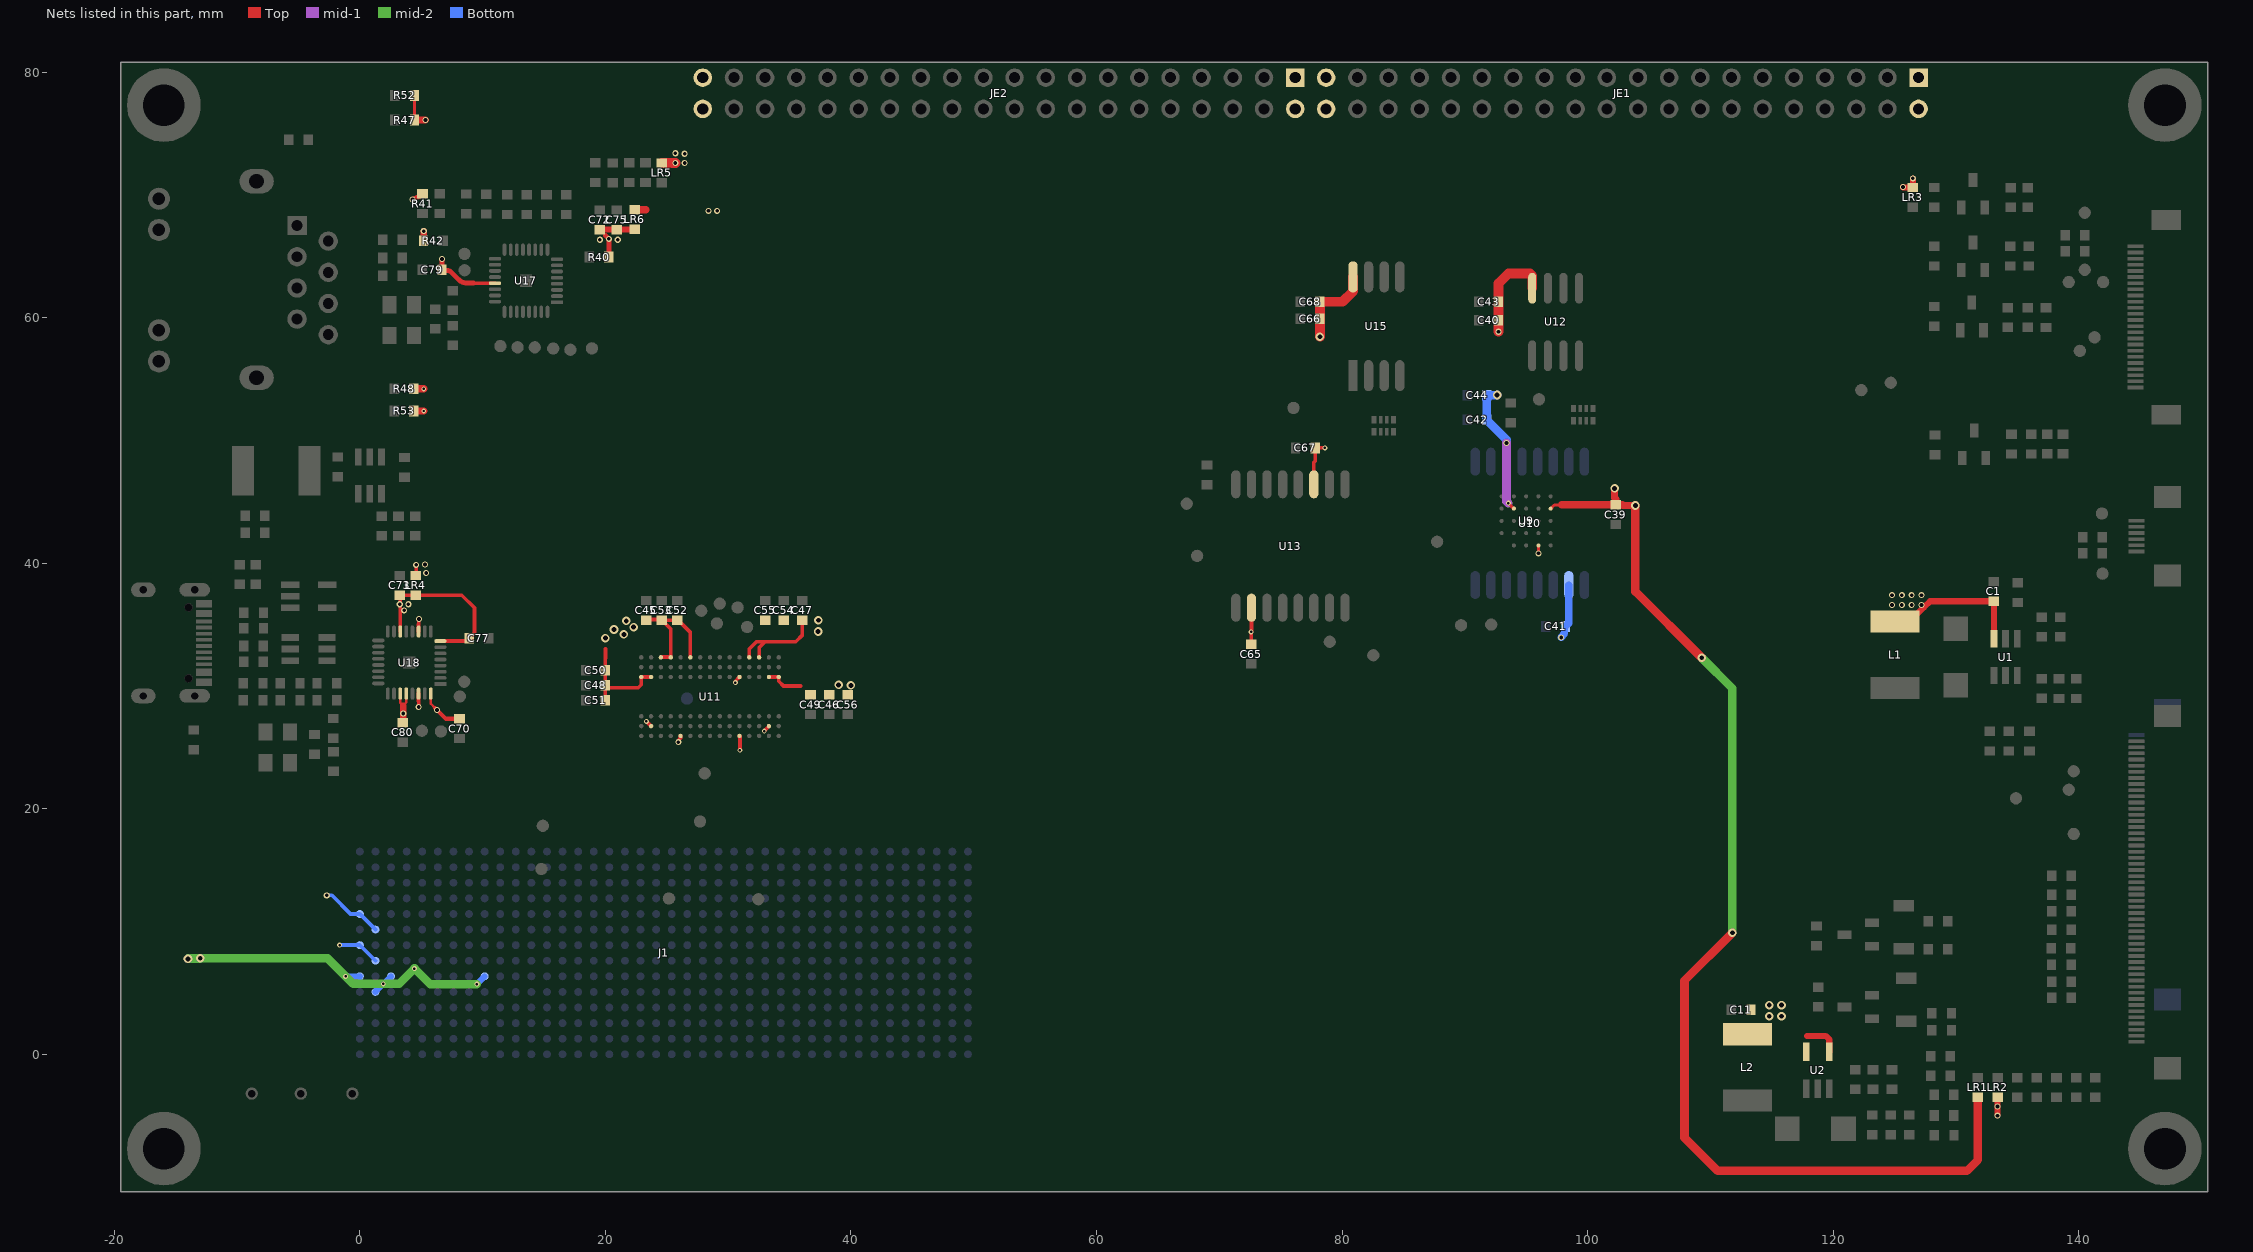
[diagram p0: the nets of this part, all layers, seen from the top]
# Altium PCB MISC105414.PcbDoc (part 3 of 11)
Units mm, origin at the board's own origin, x right, y up, seen from the top; angles counter-clockwise.
Board outline 170 x 92 mm, 6 copper layers (Top, GND, mid-1, mid-2, mid-3, Bottom), stack 1.231 mm thick; 238 components, 304 nets, 1456 pads, 1258 vias.
Unrouted connection lines stored in the file: 57.

## Footprints (in the part's own frame and the unit in brackets; to place one, negate y for a bottom-side part, rotate by r counter-clockwise, add the part's x,y. Pads: shape width x height; smd on the part's side, far side on the other; paste and mask are expansions set on the pad) (continued)
ASP-184330-01_BOTTOM [mm]
  round 0.64 smd far side: A1(0,-2.54) A2(1.27,-2.54) A3(2.54,-2.54) A4(3.81,-2.54) A5(5.08,-2.54) A6(6.35,-2.54) A7(7.62,-2.54) A8(8.89,-2.54) A9(10.16,-2.54) A10(11.43,-2.54) A11(12.7,-2.54) A12(13.97,-2.54) A13(15.24,-2.54) A14(16.51,-2.54) A15(17.78,-2.54) A16(19.05,-2.54) A17(20.32,-2.54) A18(21.59,-2.54) A19(22.86,-2.54) A20(24.13,-2.54) A21(25.4,-2.54) A22(26.67,-2.54) A23(27.94,-2.54) A24(29.21,-2.54) A25(30.48,-2.54) A26(31.75,-2.54) A27(33.02,-2.54) A28(34.29,-2.54) A29(35.56,-2.54) A30(36.83,-2.54) A31(38.1,-2.54) A32(39.37,-2.54) A33(40.64,-2.54) A34(41.91,-2.54) A35(43.18,-2.54) A36(44.45,-2.54) A37(45.72,-2.54) A38(46.99,-2.54) A39(48.26,-2.54) A40(49.53,-2.54) B1(0,-3.81) B2(1.27,-3.81) B3(2.54,-3.81) B4(3.81,-3.81) B5(5.08,-3.81) B6(6.35,-3.81) B7(7.62,-3.81) B8(8.89,-3.81) B9(10.16,-3.81) B10(11.43,-3.81) B11(12.7,-3.81) B12(13.97,-3.81) B13(15.24,-3.81) B14(16.51,-3.81) B15(17.78,-3.81) B16(19.05,-3.81) B17(20.32,-3.81) B18(21.59,-3.81) B19(22.86,-3.81) B20(24.13,-3.81) B21(25.4,-3.81) B22(26.67,-3.81) B23(27.94,-3.81) B24(29.21,-3.81) B25(30.48,-3.81) B26(31.75,-3.81) B27(33.02,-3.81) B28(34.29,-3.81) B29(35.56,-3.81) B30(36.83,-3.81) B31(38.1,-3.81) B32(39.37,-3.81) B33(40.64,-3.81) B34(41.91,-3.81) B35(43.18,-3.81) B36(44.45,-3.81) B37(45.72,-3.81) B38(46.99,-3.81) B39(48.26,-3.81) B40(49.53,-3.81) C1(0,-5.08) C2(1.27,-5.08) C3(2.54,-5.08) C4(3.81,-5.08) C5(5.08,-5.08) C6(6.35,-5.08) C7(7.62,-5.08) C8(8.89,-5.08) C9(10.16,-5.08) C10(11.43,-5.08) C11(12.7,-5.08) C12(13.97,-5.08) C13(15.24,-5.08) C14(16.51,-5.08) C15(17.78,-5.08) C16(19.05,-5.08) C17(20.32,-5.08) C18(21.59,-5.08) C19(22.86,-5.08) C20(24.13,-5.08) C21(25.4,-5.08) C22(26.67,-5.08) C23(27.94,-5.08) C24(29.21,-5.08) C25(30.48,-5.08) C26(31.75,-5.08) C27(33.02,-5.08) C28(34.29,-5.08) C29(35.56,-5.08) C30(36.83,-5.08) C31(38.1,-5.08) C32(39.37,-5.08) C33(40.64,-5.08) C34(41.91,-5.08) C35(43.18,-5.08) C36(44.45,-5.08) C37(45.72,-5.08) C38(46.99,-5.08) C39(48.26,-5.08) C40(49.53,-5.08) D1(0,-6.35) D2(1.27,-6.35) D3(2.54,-6.35) D4(3.81,-6.35) D5(5.08,-6.35) D6(6.35,-6.35) D7(7.62,-6.35) D8(8.89,-6.35) D9(10.16,-6.35) D10(11.43,-6.35) D11(12.7,-6.35) D12(13.97,-6.35) D13(15.24,-6.35) D14(16.51,-6.35) D15(17.78,-6.35) D16(19.05,-6.35) D17(20.32,-6.35) D18(21.59,-6.35) D19(22.86,-6.35) D20(24.13,-6.35) D21(25.4,-6.35) D22(26.67,-6.35) D23(27.94,-6.35) D24(29.21,-6.35) D25(30.48,-6.35) D26(31.75,-6.35) D27(33.02,-6.35) D28(34.29,-6.35) D29(35.56,-6.35) D30(36.83,-6.35) D31(38.1,-6.35) D32(39.37,-6.35) D33(40.64,-6.35) D34(41.91,-6.35) D35(43.18,-6.35) D36(44.45,-6.35) D37(45.72,-6.35) D38(46.99,-6.35) D39(48.26,-6.35) D40(49.53,-6.35) E1(0,-7.62) E2(1.27,-7.62) E3(2.54,-7.62) E4(3.81,-7.62) E5(5.08,-7.62) E6(6.35,-7.62) E7(7.62,-7.62) E8(8.89,-7.62) E9(10.16,-7.62) E10(11.43,-7.62) E11(12.7,-7.62) E12(13.97,-7.62) E13(15.24,-7.62) E14(16.51,-7.62) E15(17.78,-7.62) E16(19.05,-7.62) E17(20.32,-7.62) E18(21.59,-7.62) E19(22.86,-7.62) E20(24.13,-7.62) E21(25.4,-7.62) E22(26.67,-7.62) E23(27.94,-7.62) E24(29.21,-7.62) E25(30.48,-7.62) E26(31.75,-7.62) E27(33.02,-7.62) E28(34.29,-7.62) E29(35.56,-7.62) E30(36.83,-7.62) E31(38.1,-7.62) E32(39.37,-7.62) E33(40.64,-7.62) E34(41.91,-7.62) E35(43.18,-7.62) E36(44.45,-7.62) E37(45.72,-7.62) E38(46.99,-7.62) E39(48.26,-7.62) E40(49.53,-7.62) F1(0,-8.89) F2(1.27,-8.89) F3(2.54,-8.89) F4(3.81,-8.89) F5(5.08,-8.89) F6(6.35,-8.89) F7(7.62,-8.89) F8(8.89,-8.89) F9(10.16,-8.89) F10(11.43,-8.89) F11(12.7,-8.89) F12(13.97,-8.89) F13(15.24,-8.89) F14(16.51,-8.89) F15(17.78,-8.89) F16(19.05,-8.89) F17(20.32,-8.89) F18(21.59,-8.89) F19(22.86,-8.89) F20(24.13,-8.89) F21(25.4,-8.89) F22(26.67,-8.89) F23(27.94,-8.89) F24(29.21,-8.89) F25(30.48,-8.89) F26(31.75,-8.89) F27(33.02,-8.89) F28(34.29,-8.89) F29(35.56,-8.89) F30(36.83,-8.89) F31(38.1,-8.89) F32(39.37,-8.89) F33(40.64,-8.89) F34(41.91,-8.89) F35(43.18,-8.89) F36(44.45,-8.89) F37(45.72,-8.89) F38(46.99,-8.89) F39(48.26,-8.89) F40(49.53,-8.89) G1(0,-10.16) G2(1.27,-10.16) G3(2.54,-10.16) G4(3.81,-10.16) G5(5.08,-10.16) G6(6.35,-10.16) G7(7.62,-10.16) G8(8.89,-10.16) G9(10.16,-10.16) G10(11.43,-10.16) G11(12.7,-10.16) G12(13.97,-10.16) G13(15.24,-10.16) G14(16.51,-10.16) G15(17.78,-10.16) G16(19.05,-10.16) G17(20.32,-10.16) G18(21.59,-10.16) G19(22.86,-10.16) G20(24.13,-10.16) G21(25.4,-10.16) G22(26.67,-10.16) G23(27.94,-10.16) G24(29.21,-10.16) G25(30.48,-10.16) G26(31.75,-10.16) G27(33.02,-10.16) G28(34.29,-10.16) G29(35.56,-10.16) G30(36.83,-10.16) G31(38.1,-10.16) G32(39.37,-10.16) G33(40.64,-10.16) G34(41.91,-10.16) G35(43.18,-10.16) G36(44.45,-10.16) G37(45.72,-10.16) G38(46.99,-10.16) G39(48.26,-10.16) G40(49.53,-10.16) H1(0,-11.43) H2(1.27,-11.43) H3(2.54,-11.43) H4(3.81,-11.43) H5(5.08,-11.43) H6(6.35,-11.43) H7(7.62,-11.43) H8(8.89,-11.43) H9(10.16,-11.43) H10(11.43,-11.43) H11(12.7,-11.43) H12(13.97,-11.43) H13(15.24,-11.43) H14(16.51,-11.43) H15(17.78,-11.43) H16(19.05,-11.43) H17(20.32,-11.43) H18(21.59,-11.43) H19(22.86,-11.43) H20(24.13,-11.43) H21(25.4,-11.43) H22(26.67,-11.43) H23(27.94,-11.43) H24(29.21,-11.43) H25(30.48,-11.43) H26(31.75,-11.43) H27(33.02,-11.43) H28(34.29,-11.43) H29(35.56,-11.43) H30(36.83,-11.43) H31(38.1,-11.43) H32(39.37,-11.43) H33(40.64,-11.43) H34(41.91,-11.43) H35(43.18,-11.43) H36(44.45,-11.43) H37(45.72,-11.43) H38(46.99,-11.43) H39(48.26,-11.43) H40(49.53,-11.43) J1(0,-12.7) J2(1.27,-12.7) J3(2.54,-12.7) J4(3.81,-12.7) J5(5.08,-12.7) J6(6.35,-12.7) J7(7.62,-12.7) J8(8.89,-12.7) J9(10.16,-12.7) J10(11.43,-12.7) J11(12.7,-12.7) J12(13.97,-12.7) J13(15.24,-12.7) J14(16.51,-12.7) J15(17.78,-12.7) J16(19.05,-12.7) J17(20.32,-12.7) J18(21.59,-12.7) J19(22.86,-12.7) J20(24.13,-12.7) J21(25.4,-12.7) J22(26.67,-12.7) J23(27.94,-12.7) J24(29.21,-12.7) J25(30.48,-12.7) J26(31.75,-12.7) J27(33.02,-12.7) J28(34.29,-12.7) J29(35.56,-12.7) J30(36.83,-12.7) J31(38.1,-12.7) J32(39.37,-12.7) J33(40.64,-12.7) J34(41.91,-12.7) J35(43.18,-12.7) J36(44.45,-12.7) J37(45.72,-12.7) J38(46.99,-12.7) J39(48.26,-12.7) J40(49.53,-12.7) K1(0,-13.97) K2(1.27,-13.97) K3(2.54,-13.97) K4(3.81,-13.97) K5(5.08,-13.97) K6(6.35,-13.97) K7(7.62,-13.97) K8(8.89,-13.97) K9(10.16,-13.97) K10(11.43,-13.97) K11(12.7,-13.97) K12(13.97,-13.97) K13(15.24,-13.97) K14(16.51,-13.97) K15(17.78,-13.97) K16(19.05,-13.97) K17(20.32,-13.97) K18(21.59,-13.97) K19(22.86,-13.97) K20(24.13,-13.97) K21(25.4,-13.97) K22(26.67,-13.97) K23(27.94,-13.97) K24(29.21,-13.97) K25(30.48,-13.97) K26(31.75,-13.97) K27(33.02,-13.97) K28(34.29,-13.97) K29(35.56,-13.97) K30(36.83,-13.97) K31(38.1,-13.97) K32(39.37,-13.97) K33(40.64,-13.97) K34(41.91,-13.97) K35(43.18,-13.97) K36(44.45,-13.97) K37(45.72,-13.97) K38(46.99,-13.97) K39(48.26,-13.97) K40(49.53,-13.97) L1(0,-15.24) L2(1.27,-15.24) L3(2.54,-15.24) L4(3.81,-15.24) L5(5.08,-15.24) L6(6.35,-15.24) L7(7.62,-15.24) L8(8.89,-15.24) L9(10.16,-15.24) L10(11.43,-15.24) L11(12.7,-15.24) L12(13.97,-15.24) L13(15.24,-15.24) L14(16.51,-15.24) L15(17.78,-15.24) L16(19.05,-15.24) L17(20.32,-15.24) L18(21.59,-15.24) L19(22.86,-15.24) L20(24.13,-15.24) L21(25.4,-15.24) L22(26.67,-15.24) L23(27.94,-15.24) L24(29.21,-15.24) L25(30.48,-15.24) L26(31.75,-15.24) L27(33.02,-15.24) L28(34.29,-15.24) L29(35.56,-15.24) L30(36.83,-15.24) L31(38.1,-15.24) L32(39.37,-15.24) L33(40.64,-15.24) L34(41.91,-15.24) L35(43.18,-15.24) L36(44.45,-15.24) L37(45.72,-15.24) L38(46.99,-15.24) L39(48.26,-15.24) L40(49.53,-15.24) M1(0,-16.51) M2(1.27,-16.51) M3(2.54,-16.51) M4(3.81,-16.51) M5(5.08,-16.51) M6(6.35,-16.51) M7(7.62,-16.51) M8(8.89,-16.51) M9(10.16,-16.51) M10(11.43,-16.51) M11(12.7,-16.51) M12(13.97,-16.51) M13(15.24,-16.51) M14(16.51,-16.51) M15(17.78,-16.51) M16(19.05,-16.51) M17(20.32,-16.51) M18(21.59,-16.51) M19(22.86,-16.51) M20(24.13,-16.51) M21(25.4,-16.51) M22(26.67,-16.51) M23(27.94,-16.51) M24(29.21,-16.51) M25(30.48,-16.51) M26(31.75,-16.51) M27(33.02,-16.51) M28(34.29,-16.51) M29(35.56,-16.51) M30(36.83,-16.51) M31(38.1,-16.51) M32(39.37,-16.51) M33(40.64,-16.51) M34(41.91,-16.51) M35(43.18,-16.51) M36(44.45,-16.51) M37(45.72,-16.51) M38(46.99,-16.51) M39(48.26,-16.51) M40(49.53,-16.51) Y1(0,0) Y2(1.27,0) Y3(2.54,0) Y4(3.81,0) Y5(5.08,0) Y6(6.35,0) Y7(7.62,0) Y8(8.89,0) Y9(10.16,0) Y10(11.43,0) Y11(12.7,0) Y12(13.97,0) Y13(15.24,0) Y14(16.51,0) Y15(17.78,0) Y16(19.05,0) Y17(20.32,0) Y18(21.59,0) Y19(22.86,0) Y20(24.13,0) Y21(25.4,0) Y22(26.67,0) Y23(27.94,0) Y24(29.21,0) Y25(30.48,0) Y26(31.75,0) Y27(33.02,0) Y28(34.29,0) Y29(35.56,0) Y30(36.83,0) Y31(38.1,0) Y32(39.37,0) Y33(40.64,0) Y34(41.91,0) Y35(43.18,0) Y36(44.45,0) Y37(45.72,0) Y38(46.99,0) Y39(48.26,0) Y40(49.53,0) Z1(0,-1.27) Z2(1.27,-1.27) Z3(2.54,-1.27) Z4(3.81,-1.27) Z5(5.08,-1.27) Z6(6.35,-1.27) Z7(7.62,-1.27) Z8(8.89,-1.27) Z9(10.16,-1.27) Z10(11.43,-1.27) Z11(12.7,-1.27) Z12(13.97,-1.27) Z13(15.24,-1.27) Z14(16.51,-1.27) Z15(17.78,-1.27) Z16(19.05,-1.27) Z17(20.32,-1.27) Z18(21.59,-1.27) Z19(22.86,-1.27) Z20(24.13,-1.27) Z21(25.4,-1.27) Z22(26.67,-1.27) Z23(27.94,-1.27) Z24(29.21,-1.27) Z25(30.48,-1.27) Z26(31.75,-1.27) Z27(33.02,-1.27) Z28(34.29,-1.27) Z29(35.56,-1.27) Z30(36.83,-1.27) Z31(38.1,-1.27) Z32(39.37,-1.27) Z33(40.64,-1.27) Z34(41.91,-1.27) Z35(43.18,-1.27) Z36(44.45,-1.27) Z37(45.72,-1.27) Z38(46.99,-1.27) Z39(48.26,-1.27) Z40(49.53,-1.27)
DO-214AC [mm]
  rect 2x2 smd: 1(0,0) 2(4.6,0)
  silkscreen extent 0,-1.5 4.6,1.5
FZ_HOLE_M3.4 [mm]
  round 6 hole 3.4: 1(0,0)
FZ_TP-SMD-MINI [mm]
  round 1 smd mask+0.05: 1(0,0)
FZ_TP-VIA [mm]
  round 1 hole 0.6 mask+0.1: 1(0,0)
  silkscreen extent -0.65,-0.65 0.65,0.65
HDR2X20 [mm] "Connector; Header; 20x2 Position"
  rect 1.5x1.5 hole 0.9: 1(0,0)
  round 1.5 hole 0.9: 2(0,2.54) 3(2.54,0) 4(2.54,2.54) 5(5.08,0) 6(5.08,2.54) 7(7.62,0) 8(7.62,2.54) 9(10.16,0) 10(10.16,2.54) 11(12.7,0) 12(12.7,2.54) 13(15.24,0) 14(15.24,2.54) 15(17.78,0) 16(17.78,2.54) 17(20.32,0) 18(20.32,2.54) 19(22.86,0) 20(22.86,2.54) 21(25.4,0) 22(25.4,2.54) 23(27.94,0) 24(27.94,2.54) 25(30.48,0) 26(30.48,2.54) 27(33.02,0) 28(33.02,2.54) 29(35.56,0) 30(35.56,2.54) 31(38.1,0) 32(38.1,2.54) 33(40.64,0) 34(40.64,2.54) 35(43.18,0) 36(43.18,2.54) 37(45.72,0) 38(45.72,2.54) 39(48.26,0) 40(48.26,2.54)
  silkscreen extent -1.27,-1.27 49.53,3.81
LD-5.5mm [mm]
  rect 1.8x4 smd: 1(-2.7,0) 2(2.7,0)
  Top pour cut-out: -1.841,-1.978 -1.841,1.978 1.8,1.978 1.8,-1.978
  silkscreen extent -2.6,-2.7 2.6,2.7
LD-5.5MM [mm]
  rect 1.8x4 smd: 1(-2.7,0) 2(2.7,0)
  Top pour cut-out: -1.841,-1.978 -1.841,1.978 1.8,1.978 1.8,-1.978
  silkscreen extent -2.6,-2.7 2.6,2.7
LL-34 [mm]
  rect 0.95x1.65 smd: 1(-1.75,0) 2(1.75,0)
  Top pour cut-out: -1.2,0.9 1.2,0.9 1.2,-0.9 -1.2,-0.9
  silkscreen extent -3,-0.9 0.9,0.9
PBGA24_6X8 [mil]
  round 13 smd: A2(47.95,51.06) A3(87.32,51.06) A4(126.69,51.06) A5(166.06,51.06) B1(8.58,11.69) B2(47.95,11.69) B3(87.32,11.69) B4(126.69,11.69) B5(166.06,11.69) C1(8.58,-27.68) C2(47.95,-27.68) C3(87.32,-27.68) C4(126.69,-27.68) C5(166.06,-27.68) D1(8.58,-67.05) D2(47.95,-67.05) D3(87.32,-67.05) D4(126.69,-67.05) D5(166.06,-67.05) E1(8.58,-106.42) E2(47.95,-106.42) E3(87.32,-106.42) E4(126.69,-106.42) E5(166.06,-106.42)
  silkscreen extent -40,-194 214,139
"QFN32 5X5" [mm]
  rect 1x1 smd: 0(0,0)
  rect 0.3x1 smd: 1(-1.751,-2.528)
  oval 0.3x1 smd: 2(-1.25,-2.528) 3(-0.75,-2.528) 4(-0.25,-2.528) 5(0.25,-2.528) 6(0.75,-2.528) 7(1.25,-2.528) 8(1.75,-2.528) 17(1.8,2.528) 18(1.3,2.528) 19(0.8,2.528) 20(0.3,2.528) 21(-0.2,2.528) 22(-0.7,2.528) 23(-1.2,2.528) 24(-1.7,2.528)
  oval 1x0.3 smd: 9(2.528,-1.75) 10(2.528,-1.25) 11(2.528,-0.75) 12(2.528,-0.25) 13(2.528,0.25) 14(2.528,0.75) 15(2.528,1.25) 16(2.528,1.75) 25(-2.528,1.75) 26(-2.528,1.25) 27(-2.528,0.75) 28(-2.528,0.25) 29(-2.528,-0.25) 30(-2.528,-0.75) 31(-2.528,-1.25) 32(-2.528,-1.75)
  Top region: -1.75,1.75 1.75,1.75 1.75,-1.75 -1.25,-1.75 -1.75,-1.25
  silkscreen extent -2.6,-3.13 2.6,2.6, body extent -2.48,-2.53 2.53,2.48, height 0.93
RJ45_HR911003A [mm] "HR911003A"
  rect 1.575x1.575 hole 0.889: 1(-4.395,4.355)
  round 1.575 hole 0.889: 2(-3.125,6.895) 3(-1.855,4.355) 4(-0.585,6.895) 5(0.685,4.355) 6(1.955,6.895) 7(3.225,4.355) 8(4.495,6.895)
  round 1.8 hole 1.02: 9(-6.575,-6.895) 10(-4.035,-6.895) 11(4.135,-6.895) 12(6.675,-6.895)
  oval 2x2.8 hole 1.2 slot 2 at 90 deg: SH1(-7.995,1.055) SH2(7.995,1.055)
  silkscreen extent -7.95,-12.99 8.05,8.59
SOIC8 [mil]
  rect 100x30 smd: 1(-158.31,75)
  oval 100x30 smd: 2(-158.31,25) 3(-158.31,-25) 4(-158.31,-75) 5(158.31,-75) 6(158.31,-25) 7(158.31,25) 8(158.31,75)
  silkscreen extent -91,-100 91,100, body extent -118,-96 118,96, height 69
SOIC16 [mil]
  oval 90x30 smd: 1(-197.83,175) 2(-197.83,125) 3(-197.83,75) 4(-197.83,25) 5(-197.83,-25) 6(-197.83,-75) 7(-197.83,-125) 8(-197.83,-175) 9(197.84,-175) 10(197.84,-125) 11(197.84,-75) 12(197.84,-25) 13(197.84,25) 14(197.84,75) 15(197.84,125) 16(197.84,175)
  silkscreen extent -199,-207 134,213
SOP8 [mm]
  oval 2.5x0.65 smd: 1(-2.75,1.905) 2(-2.75,0.635) 3(-2.75,-0.635) 4(-2.75,-1.905) 5(2.75,-1.905) 6(2.75,-0.635) 7(2.75,0.635) 8(2.75,1.905)
  silkscreen extent -2.87,-2.5 0.8,2.82, body extent -2,-2.5 2,2.5, height 1.75
SOT-23 [mm]
  rect 0.7x1.15 smd: 1(-0.95,-1.125) 2(0.95,-1.125) 3(0,1.125)
  silkscreen extent -1.87,-1.23 1.5,0.7, body extent -1.5,-0.7 1.5,0.7, height 1.1
SOT-23-5 [mm]
  rect 1.5x0.52 smd: 1(-1.497,0.94) 2(-1.497,0) 3(-1.497,-0.94) 4(1.497,-0.94) 5(1.497,0.94)
  silkscreen extent -0.25,-1.41 0.25,1.41, body extent -1.45,-1.42 1.35,1.48, height 1.2
SOT-23-6 [mm]
  rect 1.4x0.55 smd: 1(0,0) 2(0,-0.95) 3(0,-1.9) 4(3,-1.9) 5(3,-0.95) 6(3,0)
  silkscreen extent -0.03,-2.5 2.01,0.63, body extent 0,-2.45 2.81,0.55, height 1.15
USB_TYPE-C_16PIN [mm]
  rect 1.3x0.6 smd mask+0.064: 1(-2.463,-3.2) 2(-2.463,-2.4) 11(-2.463,2.4) 12(-2.463,3.2)
  rect 1.3x0.3 smd mask+0.064: 3(-2.463,-1.75) 4(-2.463,-1.25) 5(-2.463,-0.75) 6(-2.463,-0.25) 7(-2.463,0.25) 8(-2.463,0.75) 9(-2.463,1.25) 10(-2.463,1.75)
  oval 2.5x1.1 hole 0.6 slot 1.6 at 0 deg: S1(-1.717,-4.32) S3(-1.717,4.32)
  oval 2x1.2 hole 0.6 slot 1.2 at 0 deg: S2(2.462,-4.32) S4(2.462,4.32)
  round 0.65 hole 0.65 unplated mask+0: ""(-1.218,2.89) ""(-1.218,-2.89)
  silkscreen extent -3.73,-4.34 5.07,4.32, body extent -2.86,-4.47 5.04,4.47, height 3.2
VFBGA90_8X13 [mil]
  round 14 smd: A1(-125.98,220.46) A2(-94.49,220.46) A3(-62.99,220.46) A7(62.99,220.46) A8(94.49,220.46) A9(125.98,220.46) B1(-125.98,188.97) B2(-94.49,188.97) B3(-62.99,188.97) B7(62.99,188.97) B8(94.49,188.97) B9(125.98,188.97) C1(-125.98,157.47) C2(-94.49,157.47) C3(-62.99,157.47) C7(62.99,157.47) C8(94.49,157.47) C9(125.98,157.47) D1(-125.98,125.98) D2(-94.49,125.98) D3(-62.99,125.98) D7(62.99,125.98) D8(94.49,125.98) D9(125.98,125.98) E1(-125.98,94.48) E2(-94.49,94.48) E3(-62.99,94.48) E7(62.99,94.48) E8(94.49,94.48) E9(125.98,94.48) F1(-125.98,62.98) F2(-94.49,62.98) F3(-62.99,62.98) F7(62.99,62.98) F8(94.49,62.98) F9(125.98,62.98) G1(-125.98,31.49) G2(-94.49,31.49) G3(-62.99,31.49) G7(62.99,31.49) G8(94.49,31.49) G9(125.98,31.49) H1(-125.98,-0.01) H2(-94.49,-0.01) H3(-62.99,-0.01) H7(62.99,-0.01) H8(94.49,-0.01) H9(125.98,-0.01) J1(-125.98,-31.5) J2(-94.49,-31.5) J3(-62.99,-31.5) J7(62.99,-31.5) J8(94.49,-31.5) J9(125.98,-31.5) K1(-125.98,-62.99) K2(-94.49,-62.99) K3(-62.99,-62.99) K7(62.99,-62.99) K8(94.49,-62.99) K9(125.98,-62.99) L1(-125.98,-94.49) L2(-94.49,-94.49) L3(-62.99,-94.49) L7(62.99,-94.49) L8(94.49,-94.49) L9(125.98,-94.49) M1(-125.98,-125.99) M2(-94.49,-125.99) M3(-62.99,-125.99) M7(62.99,-125.99) M8(94.49,-125.99) M9(125.98,-125.99) N1(-125.98,-157.48) N2(-94.49,-157.48) N3(-62.99,-157.48) N7(62.99,-157.48) N8(94.49,-157.48) N9(125.98,-157.48) P1(-125.98,-188.98) P2(-94.49,-188.98) P3(-62.99,-188.98) P7(62.99,-188.98) P8(94.49,-188.98) P9(125.98,-188.98) R1(-125.98,-220.47) R2(-94.49,-220.47) R3(-62.99,-220.47) R7(62.99,-220.47) R8(94.49,-220.47) R9(125.98,-220.47)
  silkscreen extent -167,-252 167,261, body extent -159,-244 159,254, height 150
XTAL_SMD3225 [mm]
  rect 1.4x1.15 smd: 1(-1.25,-1) 2(1.25,-1) 3(1.25,1) 4(-1.25,1)
  Top pour cut-out: -2.062,-0.292 -2.062,0.266 2.078,0.266 2.078,-0.292
  Top pour cut-out: -0.411,-1.664 -0.411,1.689 0.427,1.689 0.427,-1.664
  silkscreen extent -2.18,-2.27 2.2,1.8
XTAL_SMD3225$2F$2 [mm]
  rect 1.4x1.15 smd: 1(-1.25,-1) 2(1.25,-1) 3(1.25,1) 4(-1.25,1)
  silkscreen extent -2.18,-2.27 2.2,1.8
?#1 [mm]
  rect 1.8x2.2 smd: 0(26.55,-2.497) 0/2(-2.15,-2.497)
  rect 0.3x1.3 smd: 1(24.5,0) 2(24,0) 3(23.5,0) 4(23,0) 5(22.5,0) 6(22,0) 7(21.5,0) 8(21,0) 9(20.5,0) 10(20,0) 11(19.5,0) 12(19,0) 13(18.5,0) 14(18,0) 15(17.5,0) 16(17,0) 17(16.5,0) 18(16,0) 19(15.5,0) 20(15,0) 21(14.5,0) 22(14,0) 23(13.5,0) 24(13,0) 25(12.5,0) 26(12,0) 27(11.5,0) 28(11,0) 29(10.5,0) 30(10,0) 31(9.5,0) 32(9,0) 33(8.5,0) 34(8,0) 35(7.5,0) 36(7,0) 37(6.5,0) 38(6,0) 39(5.5,0) 40(5,0) 41(4.5,0) 42(4,0) 43(3.5,0) 44(3,0) 45(2.5,0) 46(2,0) 47(1.5,0) 48(1,0) 49(0.5,0) 50(0,0)
  silkscreen extent -2.43,-5.8 26.92,1.8
?#2 [mm]
  rect 1.8x2.2 smd: 0(-2.05,-2.497) 0/2(21.55,-2.497)
  rect 0.3x1.3 smd: 1(19.5,0) 2(19,0) 3(18.5,0) 4(18,0) 5(17.5,0) 6(17,0) 7(16.5,0) 8(16,0) 9(15.5,0) 10(15,0) 11(14.5,0) 12(14,0) 13(13.5,0) 14(13,0) 15(12.5,0) 16(12,0) 17(11.5,0) 18(11,0) 19(10.5,0) 20(10,0) 21(9.5,0) 22(9,0) 23(8.5,0) 24(8,0) 25(7.5,0) 26(7,0) 27(6.5,0) 28(6,0) 29(5.5,0) 30(5,0) 31(4.5,0) 32(4,0) 33(3.5,0) 34(3,0) 35(2.5,0) 36(2,0) 37(1.5,0) 38(1,0) 39(0.5,0) 40(0,0)
  silkscreen extent -2.43,-5.8 21.93,1.8
?#3 [mm]
  rect 1.8x2.2 smd: 0(1.95,-2.497) 0/2(-4.45,-2.497)
  rect 0.3x1.3 smd: 1(0,0) 2(-0.5,0) 3(-1,0) 4(-1.5,0) 5(-2,0) 6(-2.5,0)
  silkscreen extent -4.92,-5.8 2.43,0.56
?#4 [mm]
  rect 1.6x2.4 smd: 0(2.15,-2.497) 0/2(-13.704,-2.497)
  rect 0.3x1.3 smd: 1(0,0) 2(-0.5,0) 3(-1,0) 4(-1.5,0) 5(-2,0) 6(-2.5,0) 7(-3,0) 8(-3.5,0) 9(-4,0) 10(-4.5,0) 11(-5,0) 12(-5.5,0) 13(-6,0) 14(-6.5,0) 15(-7,0) 16(-7.5,0) 17(-8,0) 18(-8.5,0) 19(-9,0) 20(-9.5,0) 21(-10,0) 22(-10.5,0) 23(-11,0) 24(-11.5,0)
  silkscreen extent -13.93,-5.8 2.43,1.8

## Via types
v1: diameter 0.4, hole 0.2, Top to Bottom, tented top, 618 vias
v2: diameter 0.5, hole 0.3, Top to Bottom, tented top, 522 vias
v3: diameter 0.5, hole 0.3, Top to Bottom, 41 vias
v4: diameter 1, hole 0.5, Top to Bottom, tented top, 36 vias
v5: diameter 0.7, hole 0.4, Top to Bottom, tented top, 34 vias
v6: diameter 1.3, hole 1.3, Top to Bottom, tented top, 3 vias
v7: diameter 4, hole 4, Top to Bottom, tented top, 2 vias
v8: diameter 3.3, hole 3.3, Top to Bottom, tented top, 2 vias

## Nets (pads, with @x,y where several pads share a name; then routed paths per layer and width w, separated by ;. In a path a pad name is that pad's centre, name@x,y a point inside that pad or via, vN(x,y) a via of type N, cw(c..) or ccw(c..) an arc to the next point about the centre after c; other vN are vias at no path point)
+1_8V: C39.1 C40.1 C41.1 C42.2 C43.2 C44.2 C45.1 C46.2 C47.2 C48.2 C49.2 C50.2 C51.2 C52.2 C53.2 C54.2 C55.2 C56.2 C65.1 C66.1 C67.2 C68.2 J1.E39 J1.F40 J1.G39 J1.H40 JE1.39 JE1.40 JE2.1 JE2.2 LR1.2 LR4.2 LR6.2 U9.B4 U9.D1 U9.E4 U10.2 U10.11 U11.A7 U11.B2 U11.B7 U11.C9 U11.D9 U11.E1 U11.F9 U11.L1 U11.L7 U11.M9 U11.N9 U11.P2 U11.P7 U11.R7 U12.8 U13.2 U13.11 U15.8 | length 179.6
  Top w0.25: v1(93.55,44.9) U9.B4@94,44.45 ; v2(96,40.8) U9.D1@96,41.45 ; U9.E4@97,44.45 97.3,44.75 97.9,44.75
  Top w0.3: LR4.2@4.566,38.997 4.578,38.997 v2(4.578,39.864) ; C51.2@19.993,28.825 C48.2@19.993,30.06 ; 20.009,33.013 20.009,32.278 19.993,32.262 C48.2@19.993,30.06 ; v1(23.338,27.112) U11.B2@23.72,26.733 ; U11.B7@23.72,30.733 U11.A7@22.92,30.733 22.92,30.096 22.676,29.852 20.201,29.852 C48.2@19.993,30.06 ; U11.C9@24.52,32.333 24.52,32.365 U11.D9@25.273,32.365 ; U11.D9@25.32,32.333 25.32,34.635 24.872,35.083 24.872,35.134 24.641,35.365 C53.2@24.59,35.365 ; v2(25.941,25.426) 25.934,25.425 25.93,25.48 25.884,25.526 26.12,25.762 U11.E1@26.12,25.933 ; U11.F9@26.92,32.333 26.92,34.359 25.914,35.365 C53.2@24.59,35.365 ; v1(30.58,30.275) 30.58,30.393 U11.L7@30.92,30.733 ; U11.L1@30.92,25.933 30.957,25.896 v1(30.957,24.763) ; U11.M9@31.72,32.333 31.72,33.02 32.3,33.6 33,33.6 ; U11.N9@32.52,32.333 32.52,33.12 33,33.6 ; v1(32.935,26.325) 32.962,26.343 U11.P2@33.32,26.733 ; U11.P7@33.32,30.733 U11.R7@34.12,30.733 34.12,30.38 34.5,30 35.914,30 ; C47.2@36.046,35.359 36.046,34.146 35.5,33.6 33,33.6 ; C65.1@72.6,33.4 72.6,34.494 72.625,34.519 U13.2@72.625,36.375 ; U13.11@77.705,46.425 77.705,48.208 77.813,48.316 77.813,49.4 v1(78.6,49.4) ; C45.1@23.317,35.365 23.317,35.411 24.59,35.411 C53.2@24.59,35.365 ; C45.1@23.317,35.365 23.317,35.134 C45.1@23.317,35.365
  Top w0.6: LR6.2@22.4,68.8 23.3,68.8 ; 97.9,44.75 C39.1@102.3,44.75 ; v5(102.2,46.1) 102.2,45.331 102.3,45.231 C39.1@102.3,44.75 ; v5(103.9,44.7) 102.882,44.7 102.832,44.75 C39.1@102.3,44.75
  Top w0.7: v5(103.9,44.7) 103.9,37.7 v5(109.3,32.3) ; v5(111.8,9.9) 107.9,6 107.9,-6.8 110.6,-9.5 130.9,-9.5 131.8,-8.6 131.8,-4.45 LR1.2@131.8,-3.5
  Top w0.8: v5(78.2,58.45) C66.1@78.2,59.9 78.2,59.951 78.2,61.249 C68.2@78.2,61.3 80.045,61.3 80.895,62.15 U15.8@80.895,63.321 ; v2(92.75,58.85) 92.75,59.749 C40.1@92.75,59.8 92.75,62.8 93.55,63.6 95.3,63.6 95.495,63.405 U12.8@95.495,62.4
  mid-1 w0.7: v2(93.4,49.8) 93.4,45.05 v1(93.55,44.9)
  mid-2 w0.7: v5(109.3,32.3) 111.8,29.8 v5(111.8,9.9)
  Bottom w0.3: v2(-2.7,12.947) -2.279,12.947 -0.762,11.43 J1.H40@0,11.43 J1.G39@1.27,10.16 ; v1(-1.65,8.9) 0,8.9 J1.F40@0,8.89 J1.E39@1.27,7.62
  Bottom w0.6: v2(97.85,33.95) 98.119,34.287 98.119,34.85 C41.1@98.2,34.85 98.475,35.125 U10.2@98.475,38.225
  Bottom w0.7: v5(92.631,53.7) 92.605,53.675 91.831,53.675 91.831,53.655 91.8,53.624 91.8,51.751 91.8,51.649 93.395,50.054 U10.11@93.395,48.275
  other v1: 72.6,34.4
  other v2: 5.4,39.2 5.3,39.9 28.4,68.7 29.1,68.7
  other v5: 39.993,30.05 39.002,30.09 20,33.9 21.5,34.2 37.329,34.435 20.7,34.6 22.3,34.8 21.7,35.3 37.341,35.358
+1_8V_ETH: C72.1 C75.2 C79.2 LR6.1 R40.1 R41.1 R42.1 R47.1 R48.1 R52.1 R53.1 U17.21 | length 16.8
  Top w0.25: R47.1@4.443,76.103 4.443,77.157 R52.1@4.443,78.103
  Top w0.3: 9.275,62.81 U17.21@11.002,62.81
  Top w0.4: v2(4.284,69.63) 4.871,69.908 5.103,69.908 R41.1@5.103,70.089 ; v2(6.685,64.788) 6.692,64.782 C79.2@6.692,63.899 6.692,63.848 7.1,63.848 cw(c7.1,63.365) 7.441,63.706 8.046,63.101 ccw(c8.75,63.805) 8.75,62.81 9.275,62.81 ; 20,66.7 v2(20.279,66.421) R40.1@20.279,64.943
  Top w0.5: R42.1@5.177,66.262 5.2,66.262 v2(5.2,67.05) ; C72.1@19.549,67.174 C75.2@20.924,67.174 22.4,67.174 LR6.1@22.4,67.2
  Top w0.6: R53.1@4.4,52.4 v1(5.2,52.4) ; R48.1@4.4,54.2 v1(5.2,54.2) ; R47.1@4.443,76.103 4.443,76.1 v2(5.35,76.1)
  other v2: 19.55,66.35 21,66.35
+1_8V_ULPI: C70.1 C73.2 C77.2 C80.1 LR4.1 U18.8 U18.11 U18.14 U18.27 U18.28 U18.30 U18.32 | length 23.9
  Top w0.2: U18.27@3.28,29.382 3.28,28.642 3.52,28.402 3.78,28.661 U18.28@3.78,29.382 ; U18.32@5.78,29.382 5.78,28.556 v2@6.124,28.213
  Top w0.3: U18.14@3.28,34.438 3.28,37.354 C73.2@3.24,37.394 4.566,37.394 LR4.1@4.566,37.397 8.306,37.397 9.336,36.368 9.336,34.331 C77.2@8.898,33.893 8.665,33.66 U18.8@6.558,33.66 ; U18.30@4.78,29.382 4.78,29.032 v2(4.785,28.295) ; U18.11@4.78,34.438 4.78,34.788 v2(4.808,35.449)
  Top w0.35: v2@6.124,28.213 6.287,28.049 7.017,27.32 C70.1@8.117,27.32
  Top w0.5: C80.1@3.492,27.019 3.532,27.058 3.532,28.391 3.52,28.402
  other v2: 3.529,27.761 6.281,28.043 3.606,36.162 3.25,36.662 3.952,36.662
+3_3V: C1.1 C11.1 J1.C39 J1.D32 J1.D36 J1.D38 J1.D40 JE1.1 JE1.2 JE2.39 JE2.40 L1.1 L2.1 LR2.2 LR3.2 LR5.2 U1.6 U2.4 U2.5 | length 49.1
  Top w0.5: 117.9,1.5 119.397,1.5 119.69,1.207 U2.4@119.69,0.197 ; L1.1@125.05,35.25 126.25,35.25 127.4,36.4 127.9,36.9 C1.1@133.1,36.9 133.1,35.535 U1.6@133.1,33.85 ; v2(125.7,70.65) 125.7,70.606 LR3.2@126.5,70.606 ; LR3.2@126.5,70.6 LR3.2@126.5,70.606 ; v2(126.5,71.35) LR3.2@126.5,70.606 ; v2(133.4,-5) LR2.2@133.4,-3.5
  Top w0.8: LR5.2@24.6,72.6 v2(25.7,72.6)
  mid-2 w0.7: v5(-14,7.775) -13.975,7.8 -13.025,7.8 v5(-13,7.825) -2.638,7.825 v1(-1.157,6.344) -0.546,5.733 v1(1.904,5.733) 3.193,5.733 v1(4.445,6.985) 5.715,5.715 v1(9.525,5.715)
  Bottom w0.5: v1(-1.157,6.344) J1.D40@0,6.35 ; J1.C39@1.27,5.08 J1.D38@2.54,6.35 ; v1(4.445,6.985) J1.D36@5.08,6.35 ; v1(9.525,5.715) J1.D32@10.16,6.35
  other v2: 133.4,-4.25 124.8,36.6 125.6,36.6 126.4,36.6 127.2,36.6 124.8,37.4 125.6,37.4 126.4,37.4 127.2,37.4 26.45,72.6 26.45,73.35 25.7,73.4
  other v5: 114.8,3.1 115.8,3.1 114.8,4 115.8,4